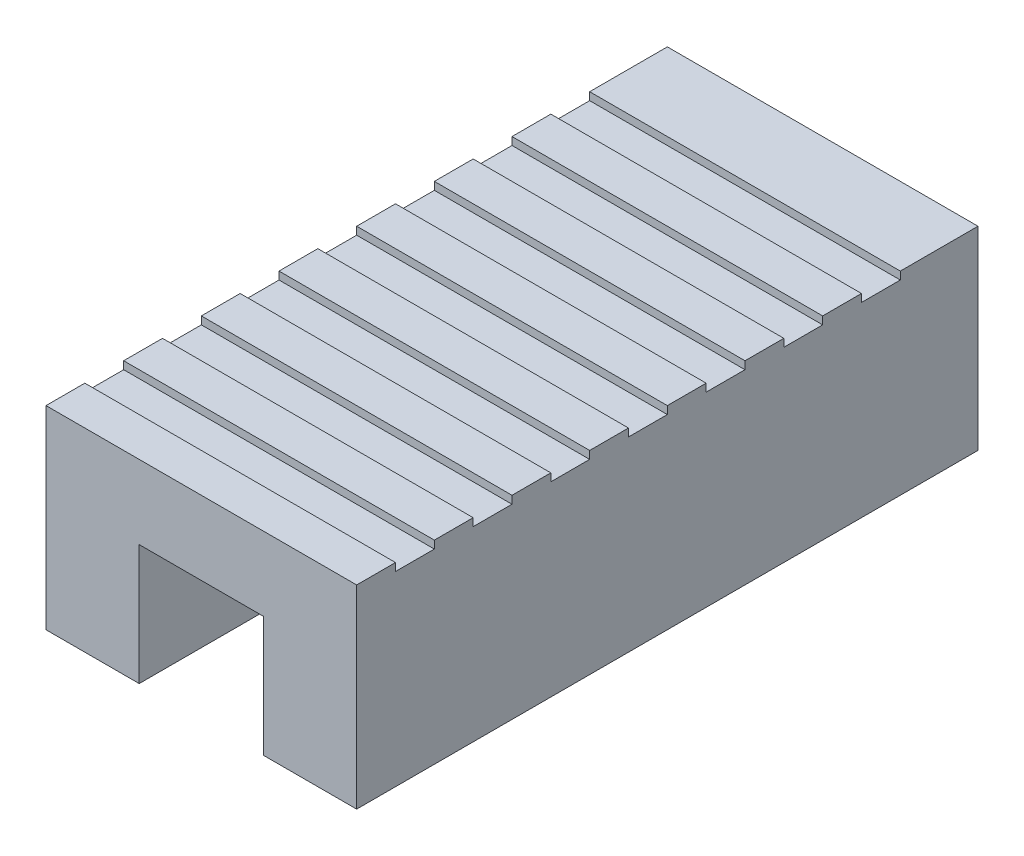
SolidWorks part; units mm, degrees
material "PE"
ref_plane "Front Plane" through (0, 0, 0) normal (0, 0, 1) x (1, 0, 0)
ref_plane "Top Plane" through (0, 0, 0) normal (0, 1, 0) x (1, 0, 0)
ref_plane "Right Plane" through (0, 0, 0) normal (1, 0, 0) x (0, 0, -1)
sketch "Sketch1" plane through (0, 0, 0) normal (0, 0, 1) x (1, 0, 0)
  line L0 (0, 25) -> (0, 6)
  line L1 (-40, 25) -> (40, 25)
  line L2 (-40, 25) -> (-40, -25)
  line L3 (-40, -25) -> (-16, -25)
  line L4 (40, 25) -> (40, -25)
  line L5 (-40, 25) -> (40, -25) construction
  line L6 (-40, -25) -> (40, 25) construction
  line L8 (-16, -25) -> (-16, 6)
  line L9 (-16, 6) -> (16, 6)
  line L10 (16, -25) -> (16, 6)
  line L11 (16, -25) -> (40, -25)
  point P0 (0, 0)
  dimension "D1" = 80
  dimension "D2" = 50
  dimension "D3" = 32
  dimension "D4" = 19
extrude "Boss-Extrude1" add sketch "Sketch1" along normal blind 160 contours L8 L9 L0 L1 L2 L3 | L10 L11 L4 L1 L0 L9
sketch "Sketch2" plane through (0, 25, 0) normal (0, 1, 0) x (1, 0, 0)
  line L0 (-40, -160) -> (-40, 0) construction
  line L1 (-40, -20) -> (40, -20)
  line L2 (-40, -20) -> (-40, -30)
  line L3 (-40, -30) -> (40, -30)
  line L4 (40, -20) -> (40, -30)
  line L5 (40, -160) -> (40, 0) construction
  line L6 (-40, 0) -> (40, 0) construction
  dimension "D1" = 20
  dimension "D2" = 10
extrude "Cut-Extrude1" cut sketch "Sketch2" against normal blind 2
pattern_linear "LPattern1" count 8 spacing 20 along (0, 0, 1) of "Cut-Extrude1"
